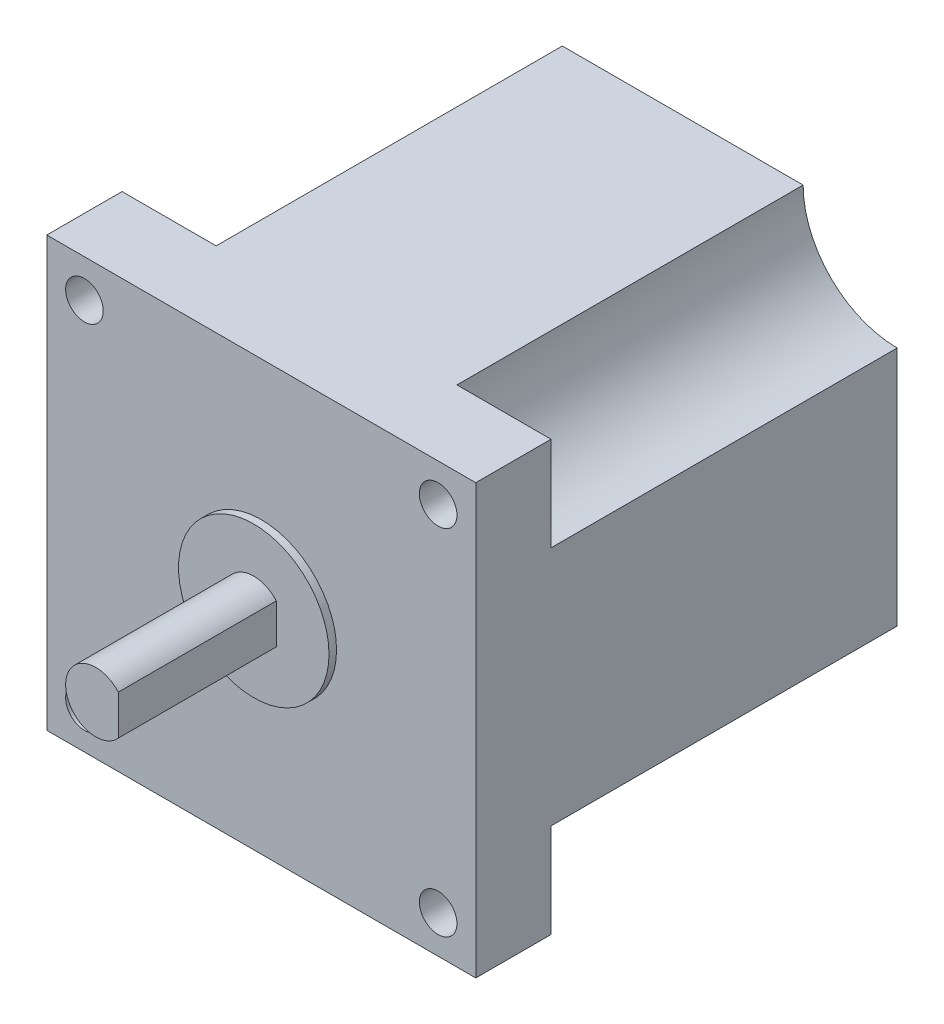
SolidWorks part; units mm, degrees
ref_plane "Front Plane" through (0, 0, 0) normal (0, 0, 1) x (1, 0, 0)
ref_plane "Top Plane" through (0, 0, 0) normal (0, 1, 0) x (1, 0, 0)
ref_plane "Right Plane" through (0, 0, 0) normal (1, 0, 0) x (0, 0, -1)
sketch "Sketch1" plane through (0, 0, 0) normal (0, 0, 1) x (1, 0, 0)
  line L1 (28.5, -28.5) -> (-28.5, -28.5)
  line L2 (28.5, -28.5) -> (28.5, 28.5)
  line L3 (28.5, 28.5) -> (-28.5, 28.5)
  line L4 (-28.5, -28.5) -> (-28.5, 28.5)
  line L5 (28.5, -28.5) -> (-28.5, 28.5) construction
  line L6 (28.5, 28.5) -> (-28.5, -28.5) construction
  point P0 (0, 0)
  dimension "D1" = 57
extrude "Boss-Extrude1" add sketch "Sketch1" along normal blind 56
sketch "Sketch2" plane through (0, 0, 56) normal (0, 0, 1) x (1, 0, 0)
  line L1 (23.5, -23.5) -> (-23.5, -23.5) construction
  line L2 (23.5, -23.5) -> (23.5, 23.5) construction
  line L3 (23.5, 23.5) -> (-23.5, 23.5) construction
  line L4 (-23.5, -23.5) -> (-23.5, 23.5) construction
  line L5 (23.5, -23.5) -> (-23.5, 23.5) construction
  line L6 (23.5, 23.5) -> (-23.5, -23.5) construction
  circle A0 centre (-23.5, 23.5) radius 2.5
  circle A1 centre (23.5, 23.5) radius 2.5
  circle A2 centre (23.5, -23.5) radius 2.5
  circle A3 centre (-23.5, -23.5) radius 2.5
  point P0 (0, 0)
  dimension "D1" = 5
  dimension "D2" = 47
extrude "Cut-Extrude1" cut sketch "Sketch2" against normal blind 98
sketch "Sketch4" plane through (0, 0, 56) normal (0, 0, 1) x (1, 0, 0)
  circle A0 centre (0, 0) radius 10
  dimension "D1" = 20
extrude "Boss-Extrude2" add sketch "Sketch4" along normal blind 1
sketch "Sketch5" plane through (0, 0, 57) normal (0, 0, 1) x (1, 0, 0)
  circle A0 centre (0, 0) radius 4
  dimension "D1" = 8
extrude "Boss-Extrude3" add sketch "Sketch5" along normal blind 21
sketch "Sketch6" plane through (0, 0, 78) normal (0, 0, 1) x (1, 0, 0)
  line L0 (3, 2.6458) -> (3, -2.6458)
  circle A0 centre (0, 0) radius 4 construction
  circle A1 centre (0, 0) radius 4
  circle M2 centre (0, 0) radius 4
  dimension "D1" = 3
extrude "Cut-Extrude2" cut sketch "Sketch6" against normal blind 21 contours L0 M2
sketch "Sketch7" plane through (0, 0, 0) normal (0, 0, -1) x (-1, 0, 0)
  line L0 (-28.5, -28.5) -> (-28.5, 28.5) construction
  line L1 (28.5, -28.5) -> (-28.5, -28.5) construction
  circle A0 centre (-28.5, 28.5) radius 12.5
  circle A1 centre (28.5, 28.5) radius 12.5
  circle A2 centre (28.5, -28.5) radius 12.5
  circle A3 centre (-28.5, -28.5) radius 12.5
  dimension "D1" = 25
extrude "Cut-Extrude3" cut sketch "Sketch7" against normal offset from surface (46 mm away) 10 up to face at (10, 0, 56)
